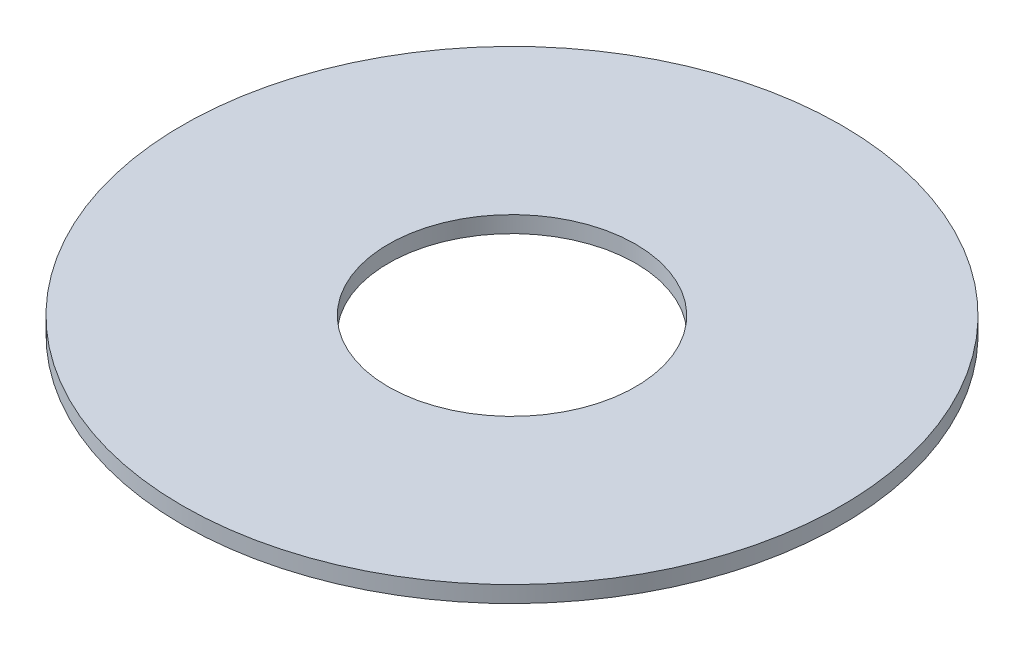
SolidWorks part; units mm, degrees
ref_plane "Front Plane" through (0, 0, 0) normal (0, 0, 1) x (1, 0, 0)
ref_plane "Top Plane" through (0, 0, 0) normal (0, 1, 0) x (1, 0, 0)
ref_plane "Right Plane" through (0, 0, 0) normal (1, 0, 0) x (0, 0, -1)
other "Configuration Table"
sketch "Sketch1" plane through (0, 0, 0) normal (0, 1, 0) x (1, 0, 0)
  circle A0 centre (0, 0) radius 22.5
  circle A1 centre (0, 0) radius 60
  dimension "D1" = 45
  dimension "D2" = 120
extrude "Boss-Extrude1" add sketch "Sketch1" along normal blind 3
